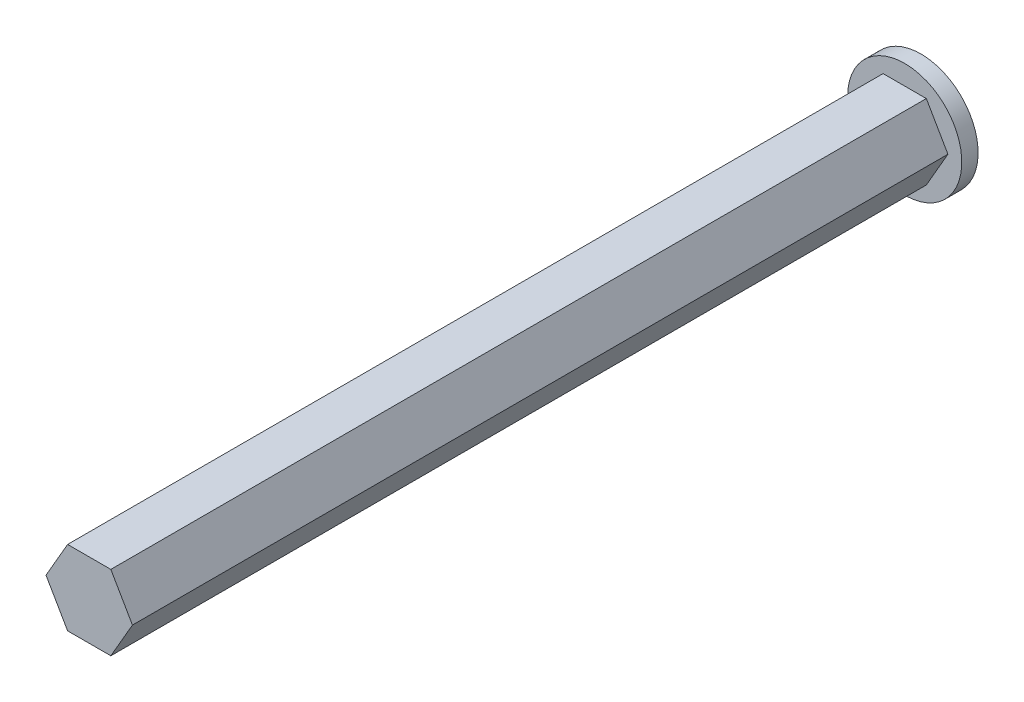
SolidWorks part; units mm, degrees
ref_plane "Front Plane" through (0, 0, 0) normal (0, 0, 1) x (1, 0, 0)
ref_plane "Top Plane" through (0, 0, 0) normal (0, 1, 0) x (1, 0, 0)
ref_plane "Right Plane" through (0, 0, 0) normal (1, 0, 0) x (0, 0, -1)
sketch "Sketch1" plane through (0, 0, 0) normal (0, 0, 1) x (1, 0, 0)
  line L1 (2.65, -4.5899) -> (5.3, 0)
  line L2 (5.3, 0) -> (2.65, 4.5899)
  line L3 (2.65, 4.5899) -> (-2.65, 4.5899)
  line L4 (-2.65, 4.5899) -> (-5.3, 0)
  line L5 (-5.3, 0) -> (-2.65, -4.5899)
  line L6 (-2.65, -4.5899) -> (2.65, -4.5899)
  circle A0 centre (0, 0) radius 4.5899 construction
  dimension "D1" = 5.3
extrude "Boss-Extrude1" add sketch "Sketch1" along normal blind 100
sketch "Sketch2" plane through (0, 0, 0) normal (0, 0, -1) x (-1, 0, 0)
  circle A0 centre (0, 0) radius 7
  dimension "D1" = 14
extrude "Boss-Extrude2" add sketch "Sketch2" along normal blind 3
chamfer "Chamfer1" distance 1 angle 60 1 edges at (-7, 0, -3)
